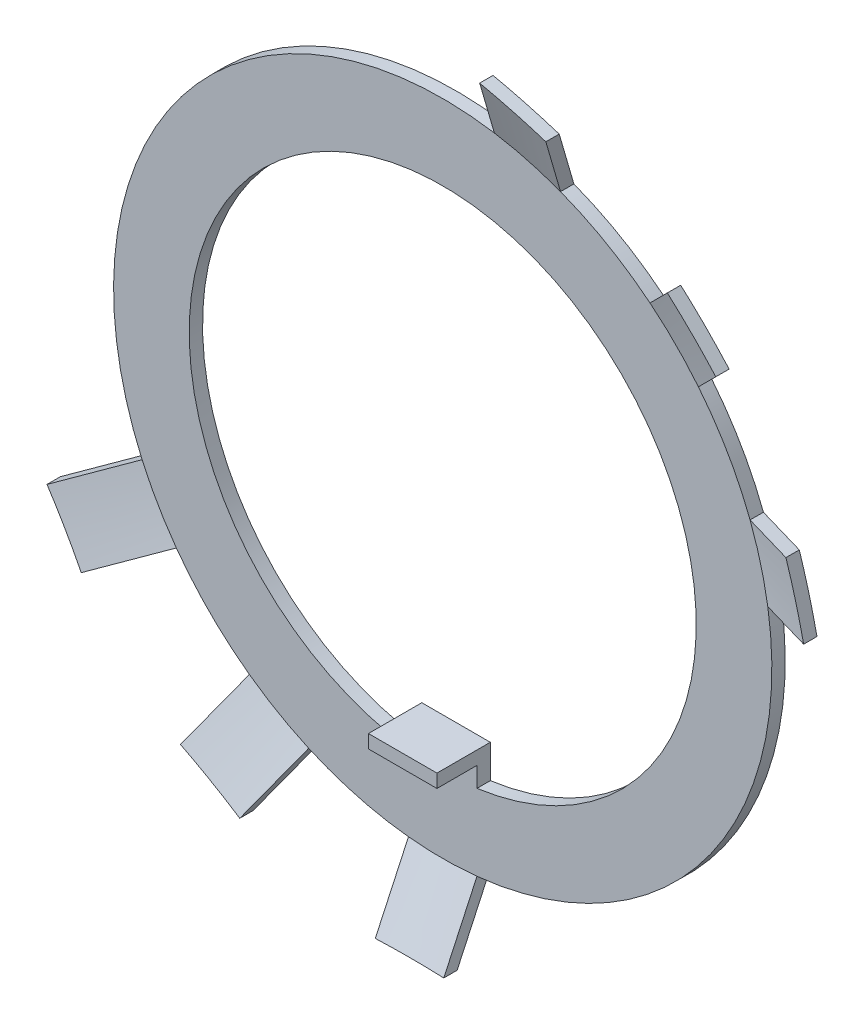
from build123d import *

# Parameters (mm, degrees)
SKETCH3_OUTSIDE_W   = 117.478
SKETCH3_OUTSIDE_H   = 117.478
CUT_EXTRUDE2_DEPTH  = 5.230463
SKETCH4_W           = 7.7
SKETCH4_H           = 1.5
BOSS_EXTRUDE1_DEPTH = 6


with BuildPart() as part:
    # Sketch2 → Base-Revolve (revolve)
    with BuildSketch(Plane(origin=(0, 0, 0), x_dir=(0, 0, -1), z_dir=(1, 0, 0))):
        Polygon((-3.730461265, 45), (0, 37), (0, 0), (-1.5, 0), (-1.5, 37), (-5.230461265, 45), align=None)
    revolve(axis=Axis((0, 0, 0), (0, 0, 1)))

    # Sketch3 outside → Cut-Extrude2 (cut)
    # profile 1 of 2: a face of its own
    with BuildSketch(Plane.XY):
        Rectangle(SKETCH3_OUTSIDE_W, SKETCH3_OUTSIDE_H)
        with BuildLine():
            Line((-3.85, -36.799150805), (-3.85, -44.835003067))
            Line((-3.85, -44.835003067), (3.85, -44.835003067))
            Line((3.85, -44.835003067), (3.85, -36.799150805))
            ThreePointArc((3.85, -36.799150805), (29.354073591, -22.524172873), (36.541703472, 5.805506641))
            Line((36.541703472, 5.805506641), (44.303740708, 7.88533825))
            Line((44.303740708, 7.88533825), (42.31083406, 15.322967112))
            Line((42.31083406, 15.322967112), (34.548796825, 13.243135503))
            ThreePointArc((34.548796825, 13.243135503), (32.04293994, 18.5), (28.743290184, 23.298567969))
            Line((28.743290184, 23.298567969), (34.425495811, 28.980773595))
            Line((34.425495811, 28.980773595), (28.980773595, 34.425495811))
            Line((28.980773595, 34.425495811), (23.298567969, 28.743290184))
            ThreePointArc((23.298567969, 28.743290184), (18.5, 32.04293994), (13.243135503, 34.548796825))
            Line((13.243135503, 34.548796825), (15.322967112, 42.31083406))
            Line((15.322967112, 42.31083406), (7.88533825, 44.303740708))
            Line((7.88533825, 44.303740708), (5.805506641, 36.541703472))
            ThreePointArc((5.805506641, 36.541703472), (-29.354073591, 22.524172873), (-33.793999435, -15.065377598))
            Line((-33.793999435, -15.065377598), (-40.753251635, -19.083303729))
            Line((-40.753251635, -19.083303729), (-36.903251635, -25.751699338))
            Line((-36.903251635, -25.751699338), (-29.943999435, -21.733773207))
            ThreePointArc((-29.943999435, -21.733773207), (-26.162950904, -26.162950904), (-21.733773207, -29.943999435))
            Line((-21.733773207, -29.943999435), (-25.751699338, -36.903251635))
            Line((-25.751699338, -36.903251635), (-19.083303729, -40.753251635))
            Line((-19.083303729, -40.753251635), (-15.065377598, -33.793999435))
            ThreePointArc((-15.065377598, -33.793999435), (-9.576304669, -35.739255573), (-3.85, -36.799150805))
        make_face(mode=Mode.SUBTRACT)
    # profile 2 of 2: a face of its own
    with BuildSketch(Plane.XY):
        with BuildLine():
            Line((3.85, -28.238758825), (3.85, -24.5))
            Line((3.85, -24.5), (-3.85, -24.5))
            Line((-3.85, -24.5), (-3.85, -28.238758825))
            ThreePointArc((-3.85, -28.238758825), (0, 28.5), (3.85, -28.238758825))
        make_face()
    extrude(amount=CUT_EXTRUDE2_DEPTH, mode=Mode.SUBTRACT)

    # Sketch4 → Boss-Extrude1 (add)
    with BuildSketch(Plane.XY):
        with Locations((0, -25.25)):
            Rectangle(SKETCH4_W, SKETCH4_H)
    extrude(amount=BOSS_EXTRUDE1_DEPTH)


solid = part.part
